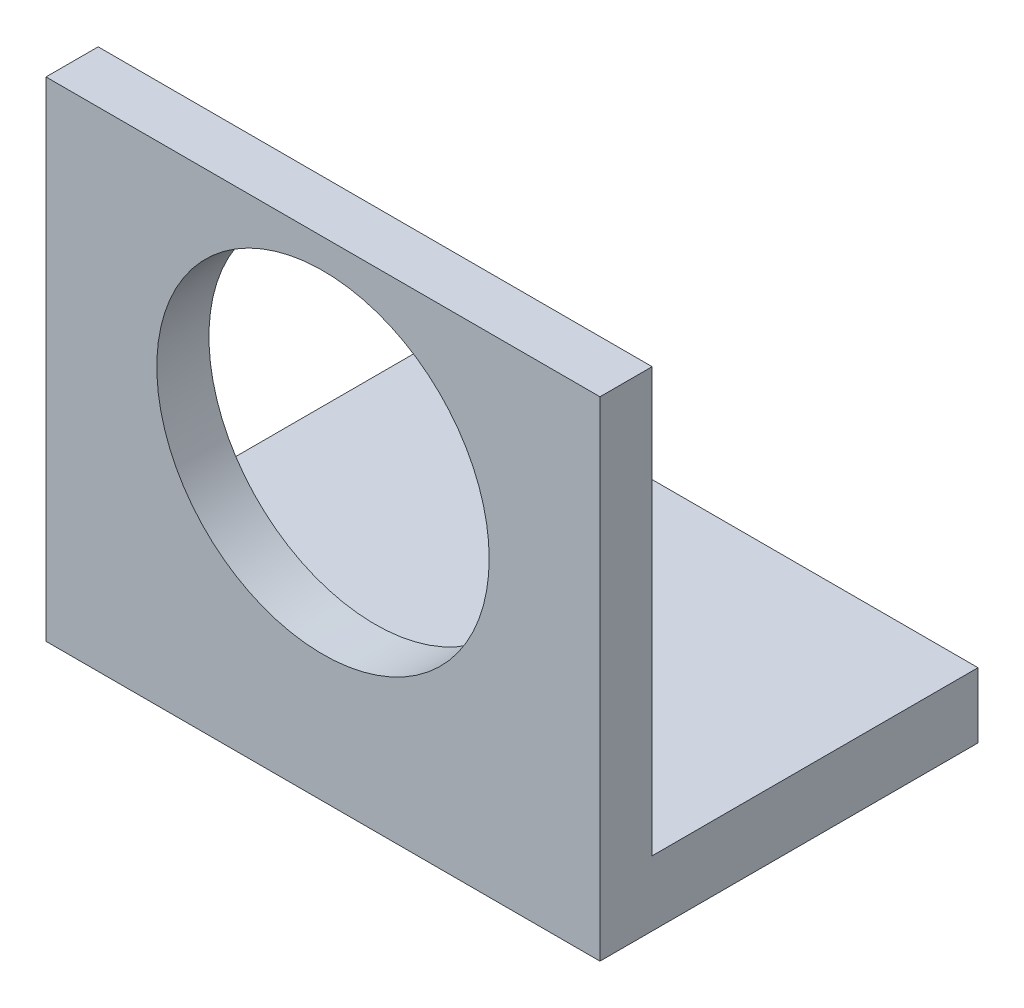
from build123d import *

# Parameters (mm, degrees)
SKETCH_1_W      = 85
SKETCH_1_H      = 75
SKETCH_1_R      = 25.5
EXTRUDE_1_DEPTH = 8
SKETCH_2_W      = 85
SKETCH_2_H      = 10
EXTRUDE_2_DEPTH = 50


with BuildPart() as part:
    # 草图1 → 凸台-拉伸1 (new body)
    with BuildSketch(Plane.XY):
        with Locations((0, -7.5)):
            Rectangle(SKETCH_1_W, SKETCH_1_H)
        Circle(SKETCH_1_R, mode=Mode.SUBTRACT)
    extrude(amount=EXTRUDE_1_DEPTH)

    # 草图2 → 凸台-拉伸2 (add)
    with BuildSketch(Plane(origin=(0, 0, 0), x_dir=(-1, 0, 0), z_dir=(0, 0, -1))):
        with Locations((0, -40)):
            Rectangle(SKETCH_2_W, SKETCH_2_H)
    extrude(amount=EXTRUDE_2_DEPTH)


solid = part.part
